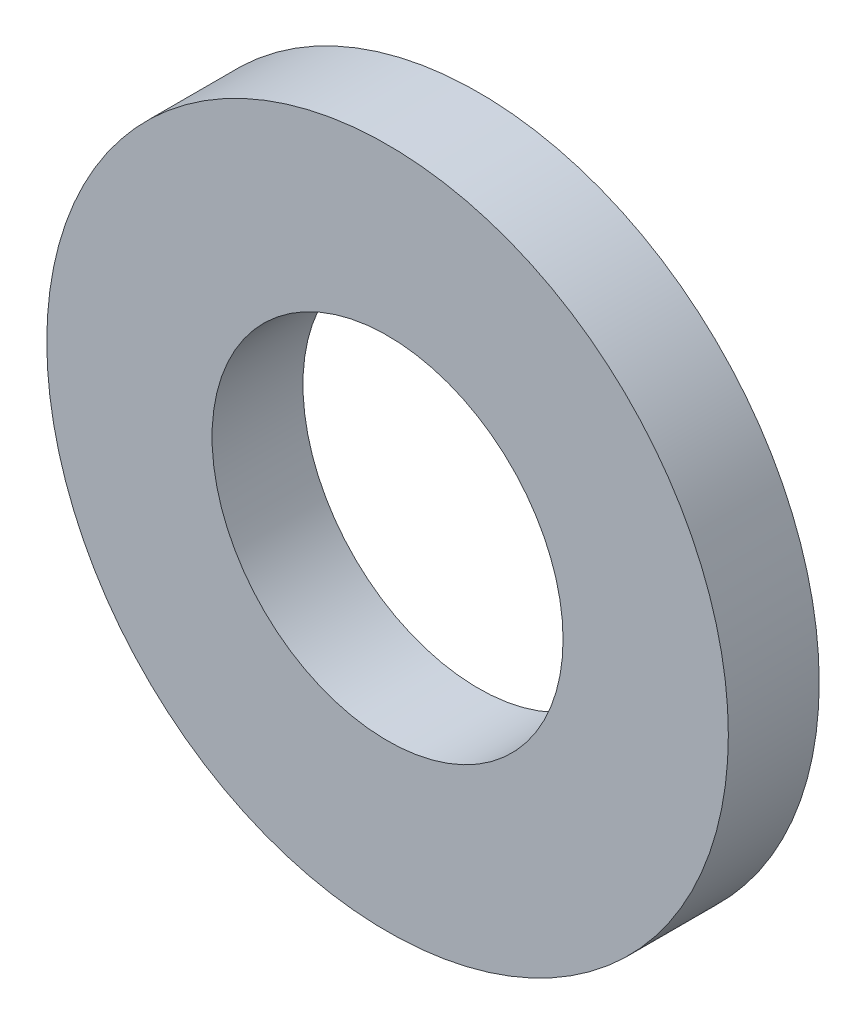
SolidWorks part; units mm, degrees
ref_plane "Front" through (0, 0, 0) normal (0, 0, 1) x (1, 0, 0)
ref_plane "Top" through (0, 0, 0) normal (0, 1, 0) x (1, 0, 0)
ref_plane "Right" through (0, 0, 0) normal (1, 0, 0) x (0, 0, -1)
other "Configuration Table"
sketch "Sketch1" plane through (0, 0, 0) normal (0, 0, 1) x (1, 0, 0)
  circle A0 centre (0, 0) radius 3.09
  circle A1 centre (0, 0) radius 6
  dimension "d1" = 6.18
  dimension "d2" = 12
extrude "Base-Extrude" add sketch "Sketch1" against normal blind 1.6
